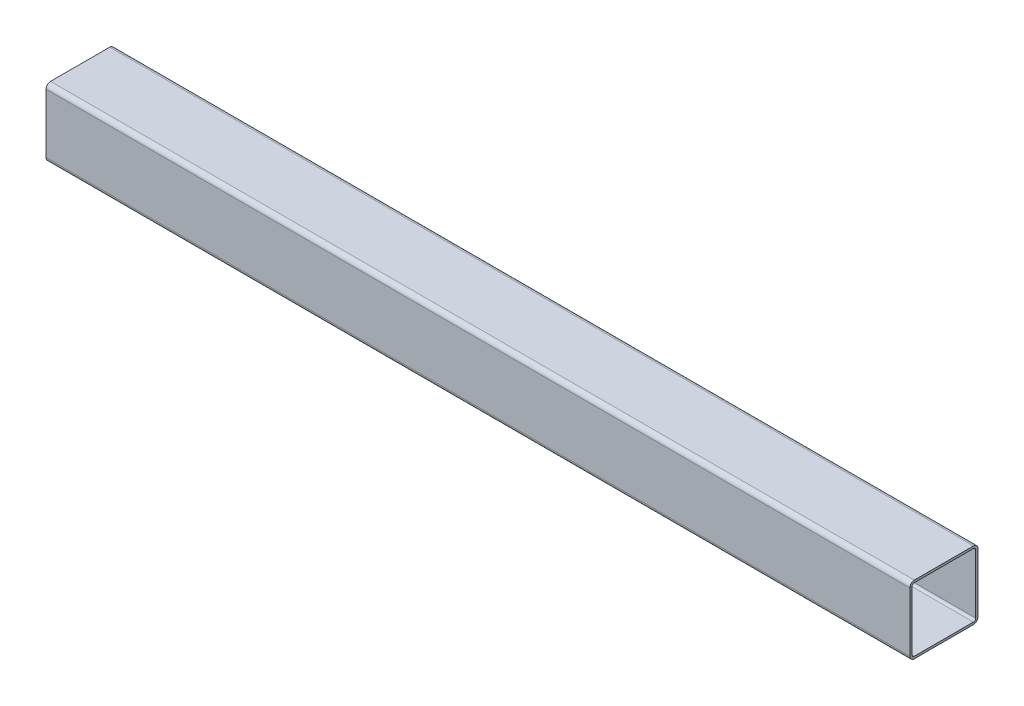
from build123d import *

# Parameters (mm, degrees)
GB_6728_1986_150_X_150_X_5_1_DEPTH = 1900


with BuildPart() as part:
    # Sketch1 → Gb／6728-1986方形空心型钢 150 X 150 X 5(1) (new body)
    with BuildSketch(Plane.YZ.offset(-950)):
        with BuildLine():
            Line((-65, -75), (65, -75))
            ThreePointArc((65, -75), (72.071067812, -72.071067812), (75, -65))
            Line((75, -65), (75, 65))
            ThreePointArc((75, 65), (72.071067812, 72.071067812), (65, 75))
            Line((65, 75), (-65, 75))
            ThreePointArc((-65, 75), (-72.071067812, 72.071067812), (-75, 65))
            Line((-75, 65), (-75, -65))
            ThreePointArc((-75, -65), (-72.071067812, -72.071067812), (-65, -75))
        make_face()
        with BuildLine():
            Line((-65, -70), (65, -70))
            ThreePointArc((65, -70), (68.535533906, -68.535533906), (70, -65))
            Line((70, -65), (70, 65))
            ThreePointArc((70, 65), (68.535533906, 68.535533906), (65, 70))
            Line((65, 70), (-65, 70))
            ThreePointArc((-65, 70), (-68.535533906, 68.535533906), (-70, 65))
            Line((-70, 65), (-70, -65))
            ThreePointArc((-70, -65), (-68.535533906, -68.535533906), (-65, -70))
        make_face(mode=Mode.SUBTRACT)
    extrude(amount=GB_6728_1986_150_X_150_X_5_1_DEPTH)


solid = part.part
